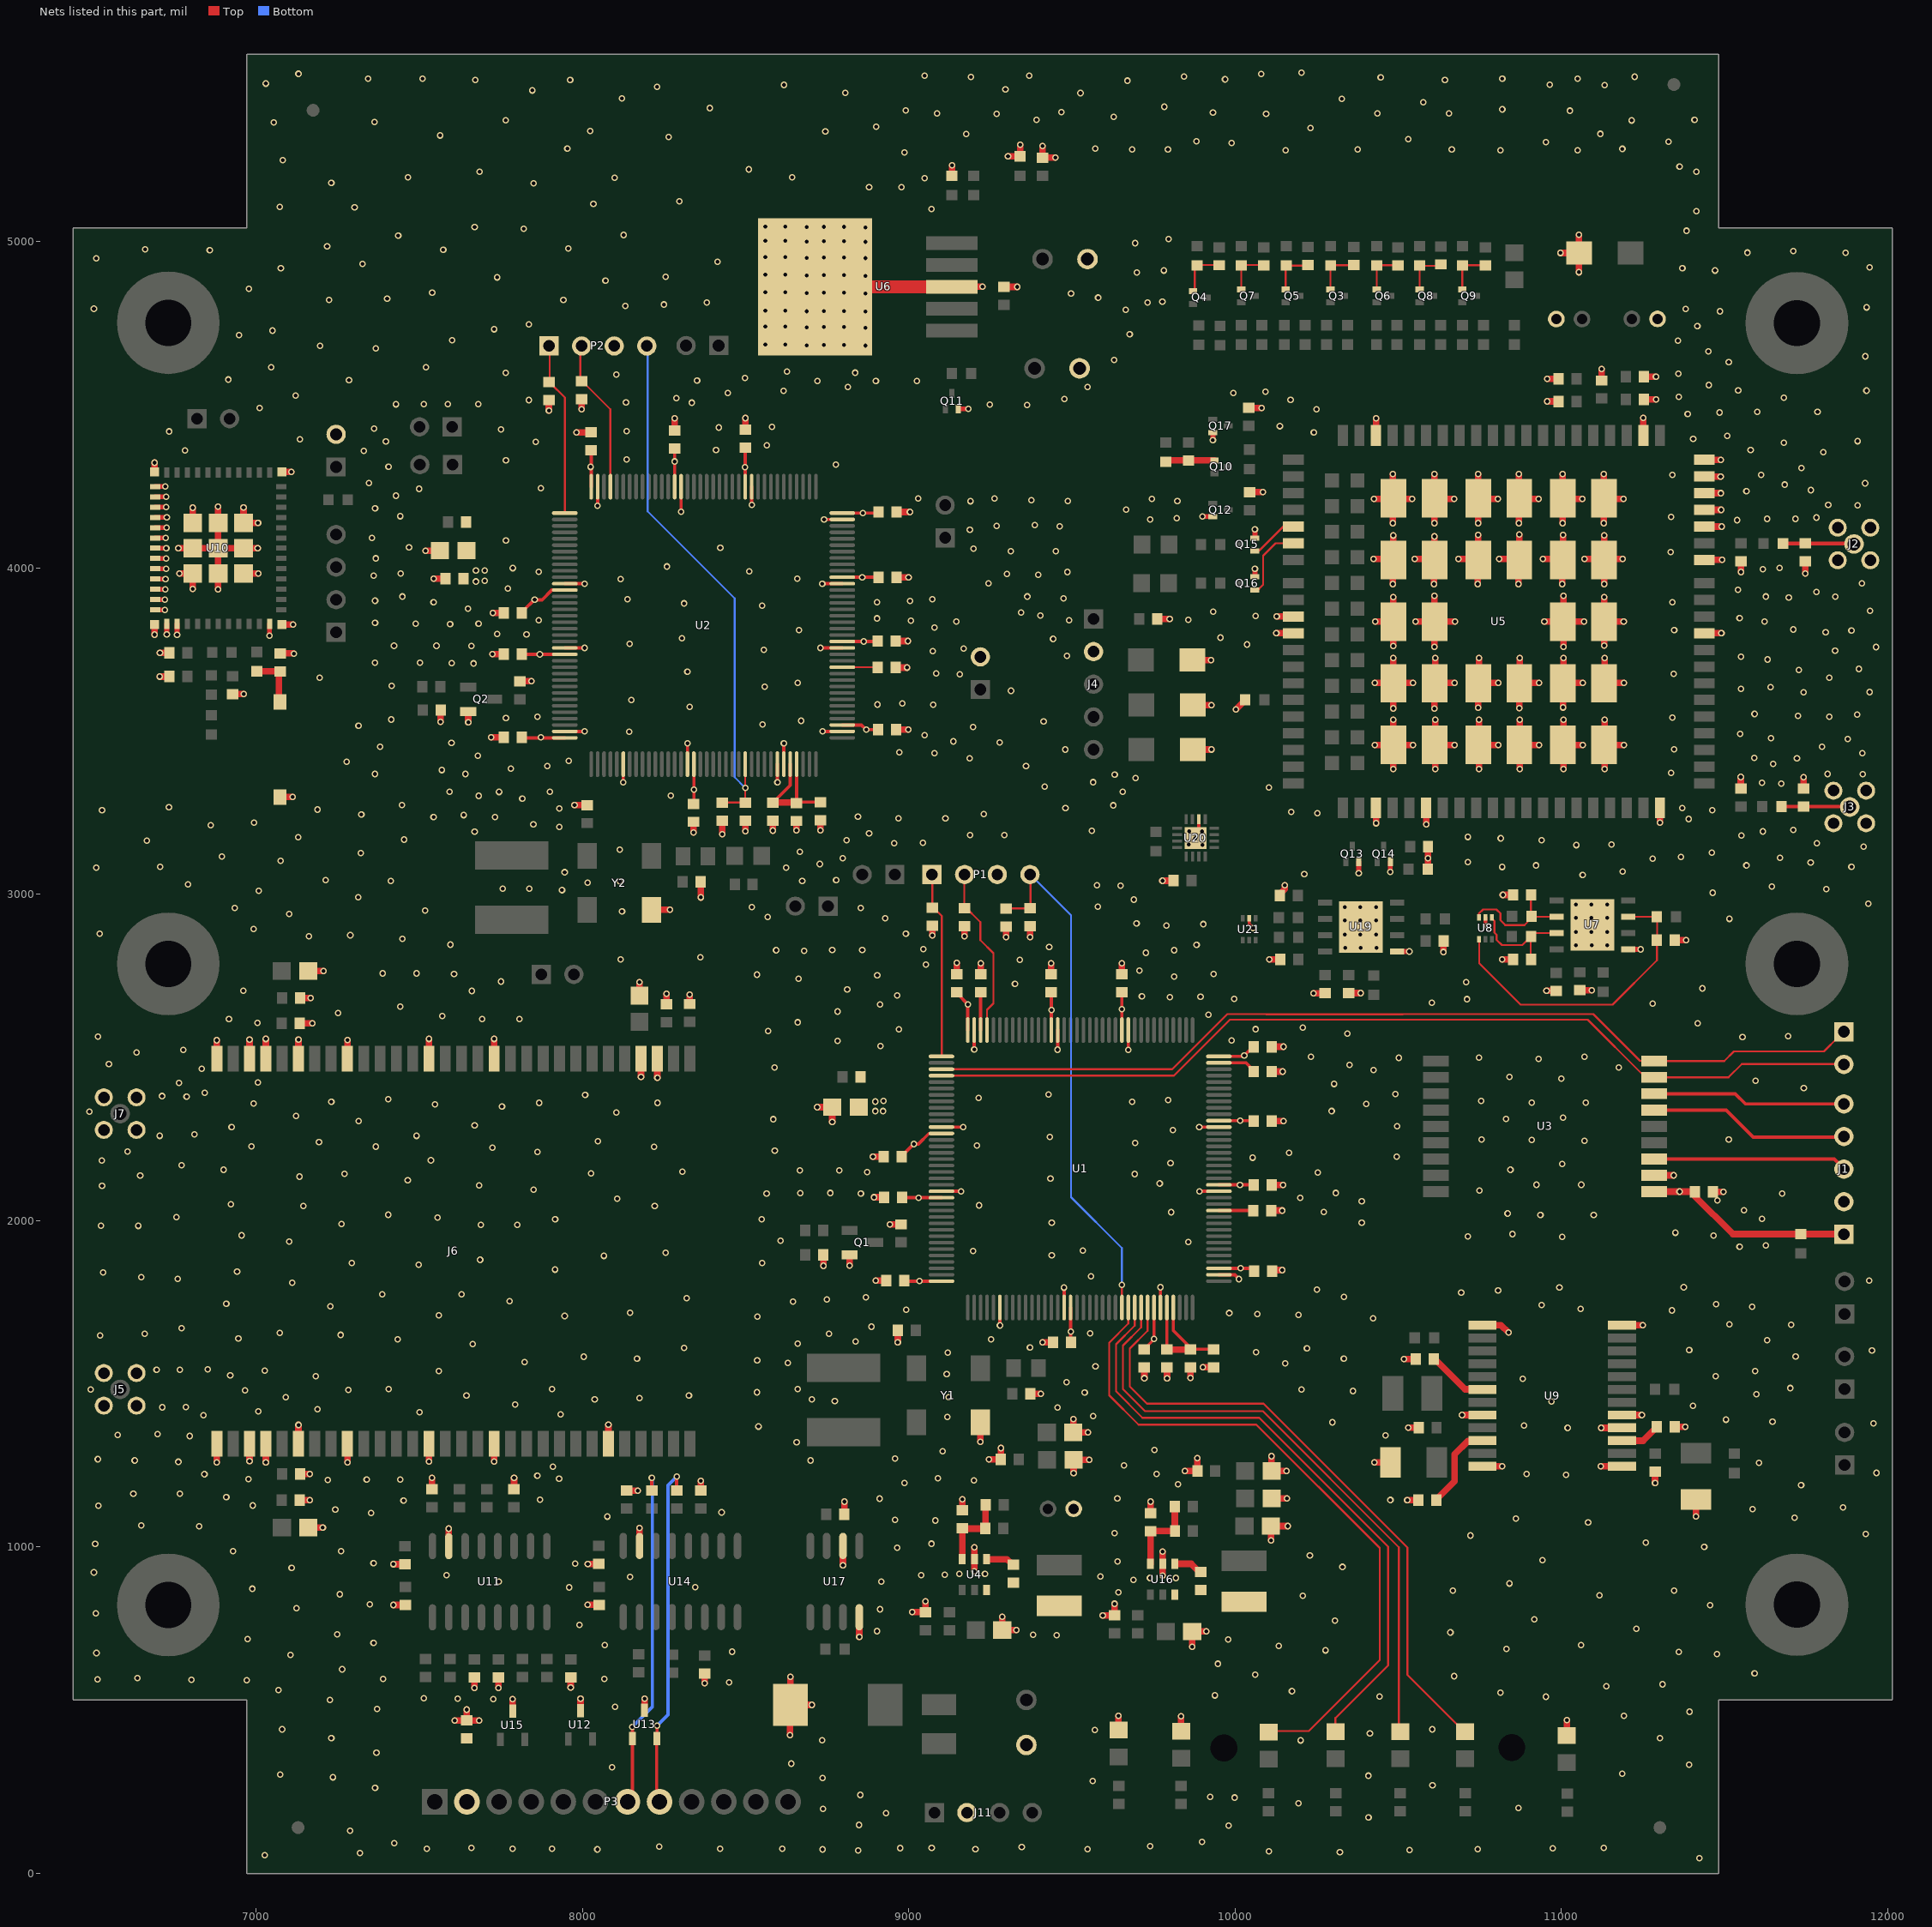
[diagram p0: the nets of this part, all layers, seen from the top]
# Altium PCB MISC86294.PcbDoc (part 5 of 8)
Units mil, origin at the board's own origin, x right, y up, seen from the top; angles counter-clockwise.
Board outline 5574.84 x 5574.84 mil, 4 copper layers (Top, GND02, PWR03, Bottom), stack 23.756 mil thick; 313 components, 311 nets, 1350 pads, 1701 vias.

## Via types
v1: diameter 20, hole 12, Top to Bottom, 1701 vias

## Nets (pads, with @x,y where several pads share a name; then routed paths per layer and width w, separated by ;. In a path a pad name is that pad's centre, name@x,y a point inside that pad or via, vN(x,y) a via of type N, cw(c..) or ccw(c..) an arc to the next point about the centre after c; other vN are vias at no path point) (continued)
GND: (continued)
  other v1: 11423,46 7026,55 7318,62 10321,65 10104,67 8845,70 10535,71 8045,73 8735,73 9204,74 9548,74 10744,74 7522,75 7785,75 7906,75 8421,75 8612,75 10974,76 8973,77 7659,78 9070,78 11130,78 9346,80 8235,82 9740,83 7423,92 9899,96 7287,130 9980,146 8847,148 10409,171 8930,184 8737,197 10868,200 10194,214 9998,232 9924,234 8851,240 7364,262 10605,270 9563,283 8735,292 7235,294 10408,299 7073,302 11186,305 8090,325 11391,333 8640,336 7368,369 10201,407 8734,408 7230,414 11302,414 10413,429 9570,439 7079,441 10604,441 11192,482 11393,495 7370,503 8099,510 7226,531 7726,534 7617,535 7513,536 10953,541 10443,542 9938,545 10813,553 10174,558 7068,561 11138,573 11310,579 8449,585 6971,592 6801,593 6513,594 7388,595 8067,595 6635,598 10671,604 10061,609 11592,613 7263,625 9947,642 7105,669 11477,672 6510,675 11360,678 8458,679 10277,683 10832,687 10134,697 8068,699 11060,699 7359,706 9979,716 6973,718 9453,730 9381,731 7248,732 10660,738 8902,742 11230,749 7990,761 10306,774 10917,778 6508,797 8912,809 7123,812 11456,821 7348,824 10207,850 11117,852 7256,855 9642,861 10667,866 11345,866 6988,872 7959,876 8345,877 10841,888 7743,894 8916,894 9688,899 9739,905 9818,905 8145,908 9587,910 7583,913 9038,913 9110,915 9155,917 9233,917 6502,922 7108,936 10329,939 7977,949 7359,950 9640,956 10942,959 10229,974 6929,987 7260,987 8964,998 11438,1000 6506,1009 9069,1010 11259,1013 10721,1035 11933,1040 9630,1042 6825,1063 6647,1066 11082,1075 9081,1081 8958,1083 10861,1087 11715,1090 8076,1093 7352,1104 8426,1106 7242,1115 11586,1116 11863,1121 6516,1126 6989,1127 7451,1142 10476,1144 7869,1145 8910,1148 9639,1149 6908,1153 6623,1163 6766,1163 11735,1189 9825,1192 8987,1196 9199,1204 7219,1205 7338,1207 7441,1207 6976,1208 7928,1209 9089,1210 7861,1218 11014,1221 6841,1223 9759,1224 10893,1224 11966,1227 7909,1246 9659,1250 11606,1258 6761,1261 6627,1265 8699,1265 6514,1269 8958,1271 9103,1293 9753,1297 8656,1321 6796,1340 10461,1342 6575,1343 6697,1346 11019,1365 8539,1369 10886,1372 11957,1379 10298,1382 11647,1384 11504,1390 9118,1398 9565,1401 6838,1404 7933,1406 7500,1413 7006,1416 7187,1422 9456,1427 6712,1428 6784,1429 11403,1433 7793,1437 10970,1446 8773,1447 8037,1452 8703,1452 8174,1456 7090,1459 9122,1459 7644,1464 8326,1464 11598,1468 9539,1473 8534,1474 10361,1478 6965,1480 7282,1481 6492,1483 10203,1483 7406,1484 7906,1484 8659,1484 11702,1487 9483,1505 10882,1515 7182,1523 11473,1523 6920,1526 9116,1530 7559,1539 11594,1539 7026,1540 6694,1543 6766,1543 6851,1544 9572,1554 10153,1563 8629,1564 7822,1567 8535,1572 8167,1577 10333,1577 8003,1583 11718,1584 9119,1596 10064,1597 11952,1602 11392,1603 10220,1609 8311,1610 9371,1611 7663,1622 8659,1623 8837,1630 11631,1634 7433,1636 9252,1636 6945,1639 6521,1648 7258,1650 6658,1653 8755,1653 9556,1655 7072,1656 6771,1670 8885,1675 11704,1681 11515,1682 10423,1701 8536,1706 7945,1708 7559,1710 10194,1711 10068,1714 9982,1717 8145,1718 11339,1725 8992,1727 11059,1730 11585,1736 7227,1737 10939,1741 11474,1744 6908,1745 8645,1752 7776,1753 8749,1759 8319,1762 8868,1765 10334,1766 7386,1774 7629,1774 10693,1780 10806,1786 10251,1789 10994,1795 11375,1796 7110,1810 11943,1816 6759,1822 6647,1827 9558,1830 6530,1841 6941,1844 7915,1850 7498,1865 7293,1870 8550,1870 7686,1880 8065,1892 9438,1894 8255,1902 9197,1907 9533,1908 11546,1920 11627,1924 9856,1935 7101,1936 8607,1939 11002,1950 10713,1952 11466,1954 6955,1955 10850,1959 11349,1963 6638,1984 6524,1985 7688,1987 7800,1987 7261,1990 9438,1994 10388,1994 7916,2004 8549,2004 11615,2006 7555,2010 6755,2011 10936,2017 11099,2017 7404,2018 10835,2022 9804,2026 10272,2027 11560,2032 7144,2045 8221,2045 9215,2047 6922,2050 10388,2059 11478,2062 8106,2067 10199,2070 8564,2083 8853,2083 11677,2083 8667,2084 8759,2085 10309,2085 10749,2092 7850,2095 6527,2107 7683,2108 10924,2110 11061,2110 9769,2114 7464,2124 9434,2129 7132,2135 6644,2138 9692,2143 7270,2144 8026,2145 10253,2148 8872,2149 8306,2150 8666,2154 8787,2154 6900,2156 10844,2156 6771,2170 11002,2174 9802,2176 6526,2184 7535,2185 10054,2193 10495,2196 10165,2208 7862,2211 6605,2212 8589,2215 7724,2224 8219,2226 7366,2227 6985,2228 9209,2230 9694,2238 7192,2241 8047,2243 11071,2245 10909,2247 10755,2249 11513,2249 9432,2257 6704,2260 7491,2260 6810,2264 9809,2278 6924,2287 10496,2289 7669,2292 7314,2305 8584,2311 10830,2312 11005,2316 7122,2321 8103,2331 6488,2334 10296,2336 7753,2350 7547,2356 10402,2358 6992,2359 7867,2361 8230,2361 10909,2362 11075,2362 7230,2364 9684,2364 10754,2367 9795,2370 7404,2372 9214,2376 6786,2380 6711,2382 8008,2385 9428,2387 10491,2388 6842,2392 11743,2406 10303,2419 6763,2422 7005,2423 11595,2429 11000,2435 10841,2441 10424,2462 6833,2466 8588,2469 11176,2470 10351,2477 6548,2480 10930,2496 10502,2499 10747,2500 10232,2502 11071,2502 6633,2515 6776,2523 8913,2535 8781,2551 9989,2552 11555,2563 6515,2564 11695,2565 10344,2573 8569,2581 8969,2586 10063,2587 10207,2592 11418,2605 7003,2606 8659,2608 6916,2618 7692,2618 7806,2618 7570,2627 9918,2631 7250,2636 8781,2641 7441,2656 8912,2663 11280,2665 10603,2668 10711,2679 9997,2680 9800,2685 9894,2686 9714,2688 8964,2690 7660,2704 6960,2705 8811,2709 11432,2712 9325,2726 10708,2731 7750,2733 8662,2742 9813,2748 8903,2752 8534,2754 7606,2756 9934,2756 7387,2758 7491,2758 9707,2767 9052,2785 9340,2799 8116,2801 8361,2807 9726,2821 8679,2827 8593,2829 9813,2829 8765,2830 8857,2830 9044,2832 10337,2836 10385,2836 10433,2836 9430,2839 11045,2844 11093,2844 11141,2844 9882,2845 7595,2846 7448,2864 7161,2872 7288,2875 10336,2877 10384,2877 10432,2877 6520,2880 8991,2880 11044,2885 11092,2885 11140,2885 6992,2894 9789,2904 9903,2909 9698,2911 10336,2920 10384,2920 10432,2920 11515,2925 8927,2927 11044,2928 11092,2928 11140,2928 8567,2931 7101,2940 8121,2948 7517,2951 6934,2958 8852,2958 8519,2961 10336,2961 10384,2961 10432,2961 9579,2962 11044,2969 11092,2969 11140,2969 11941,2972 9690,2984 7312,2991 11464,3005 7007,3011 7937,3013 11812,3016 7837,3017 7755,3018 11645,3024 9649,3027 9577,3028 6790,3031 8015,3036 8114,3040 7412,3041 8673,3041 7212,3044 8777,3044 11065,3060 10212,3062 7945,3068 11188,3070 6509,3082 8624,3082 10818,3084 6705,3085 11889,3085 10922,3089 11567,3089 8727,3093 11764,3098 10713,3099 7074,3103 11280,3110 8797,3111 11670,3112 11366,3115 6894,3116 7320,3127 11461,3128 8666,3131 8114,3137 11926,3146 11046,3151 9900,3152 9858,3153 11154,3153 8955,3157 11783,3157 9043,3158 6664,3165 8809,3166 10939,3166 7453,3168 9878,3172 10814,3172 7128,3175 10713,3176 11552,3180 9188,3182 9293,3182 8878,3187 7669,3192 9898,3193 11618,3193 9859,3194 9561,3195 11711,3198 7929,3207 6860,3212 7849,3215 6993,3220 11390,3231 8968,3233 9112,3233 7543,3237 7731,3237 8844,3238 7636,3243 7322,3245 9230,3246 10252,3249 10172,3253 6527,3258 11462,3258 7187,3260 7929,3263 9480,3265 11370,3265 6732,3267 9626,3273 7446,3274 7815,3293 7682,3302 8270,3303 7744,3314 7592,3315 7900,3315 9655,3315 10104,3328 9416,3330 11674,3339 11615,3342 9565,3344 9695,3357 9631,3367 11924,3368 7363,3369 7641,3369 11816,3369 11336,3372 7568,3381 7780,3385 7892,3393 9359,3393 11649,3400 7277,3406 7957,3409 9186,3417 11722,3417 11591,3418 7679,3425 9079,3433 11922,3433 8971,3435 9479,3444 11345,3445 7379,3452 11799,3453 7598,3464 9278,3466 9136,3469 11878,3476 11642,3479 9048,3488 11548,3492 8143,3499 9197,3513 7313,3517 8552,3521 9413,3530 8670,3532 7413,3536 7765,3541 11340,3542 7862,3545 11821,3545 11725,3547 11907,3551 11592,3553 8328,3575 9075,3581 8904,3582 8980,3585 8149,3596 11742,3619 11945,3620 9313,3624 11550,3630 11641,3635 8558,3637 7415,3639 8659,3648 7194,3664 11821,3664 9156,3675 11344,3676 9084,3677 8321,3682 11728,3688 11912,3691 7666,3708 7599,3709 7363,3710 7501,3710 11632,3720 11550,3728 9485,3731 7115,3738 9073,3746 11839,3747 8555,3749 9168,3753 11964,3758 7659,3761 7422,3762 7552,3762 10037,3766 8144,3768 9442,3783 8304,3785 9955,3787 7828,3797 7738,3798 11810,3803 11889,3809 8663,3810 11346,3810 11711,3812 9078,3818 7594,3828 7488,3830 7681,3830 7364,3832 9146,3836 11623,3836 9006,3839 7866,3840 9491,3840 9856,3841 8902,3846 11546,3847 10063,3853 9403,3855 9344,3864 9933,3866 11946,3869 7649,3876 8550,3885 8311,3892 7543,3895 8902,3895 11340,3895 9004,3899 7364,3900 8138,3905 9072,3905 9474,3907 11697,3910 11840,3912 7448,3913 9363,3913 11627,3913 11782,3927 11541,3934 7771,3937 9244,3953 11921,3953 8116,3966 8658,3968 7360,3977 9397,3980 9301,3982 7442,3983 9486,3988 7865,3989 8511,3990 11617,3997 7786,4000 11669,4001 8258,4005 7366,4030 11335,4049 9312,4052 9450,4052 9198,4060 8422,4062 7468,4064 7765,4085 7354,4093 9187,4117 9462,4128 9269,4129 9386,4132 11539,4147 9740,4149 11631,4151 11717,4151 9821,4153 11782,4155 11336,4157 7441,4159 9666,4179 7364,4183 11908,4192 11818,4194 9189,4205 9487,4206 9823,4206 9376,4208 9745,4212 9029,4213 9262,4213 7428,4222 11567,4236 11765,4239 7499,4243 7872,4245 11685,4256 11931,4260 7345,4261 11340,4286 11612,4286 11736,4307 7405,4311 8776,4317 7765,4330 8135,4333 11803,4355 7329,4359 6781,4361 8409,4362 11580,4362 8565,4376 11682,4384 7856,4387 7397,4388 11908,4389 7134,4395 11404,4396 11508,4405 10241,4416 6733,4419 8135,4420 7750,4425 7361,4428 8417,4431 8580,4433 10137,4435 11387,4472 11485,4477 11600,4479 11785,4479 10249,4487 7010,4491 9362,4500 9248,4501 7428,4502 7513,4503 7587,4503 7680,4503 8335,4507 8133,4508 7835,4515 10170,4516 9477,4518 8287,4521 11682,4522 11360,4525 7120,4529 8445,4537 9994,4537 10093,4541 8616,4543 11935,4544 11542,4545 8813,4555 9548,4555 11452,4561 8720,4574 8899,4574 9025,4574 8351,4575 7284,4576 6914,4578 8498,4583 8103,4593 11359,4596 7764,4598 8835,4599 8626,4602 7045,4616 7520,4616 11513,4631 9629,4638 11932,4649 11451,4664 7366,4673 7195,4681 8867,4682 8687,4683 8740,4684 8801,4684 8560,4685 8621,4685 11357,4697 7600,4698 6947,4714 9677,4717 7049,4728 7729,4732 8867,4737 8687,4738 8740,4739 8801,4739 8560,4740 8621,4740 11417,4742 7835,4747 8867,4786 8687,4787 11486,4787 8740,4788 8801,4788 8560,4789 8621,4789 9665,4792 11381,4794 6502,4795 11936,4799 8131,4803 8249,4808 8381,4814 9732,4814 9777,4817 7223,4822 7941,4822 7401,4826 9580,4829 8867,4842 9497,4842 8687,4843 7539,4844 8740,4844 8801,4844 8560,4845 8621,4845 6977,4856 8070,4881 7738,4891 8254,4893 8867,4896 8687,4897 8740,4898 8801,4898 8560,4899 8621,4899 9699,4906 9782,4912 11471,4912 7075,4919 11371,4919 11945,4922 7325,4932 8414,4939 6509,4949 8867,4950 8687,4951 8740,4952 8801,4952 8560,4953 8621,4953 11871,4966 11570,4967 11711,4972 6857,4974 7573,4976 6659,4977 7956,4980 7217,4986 9694,4996 8867,5000 8687,5001 8740,5002 8801,5002 8560,5003 8621,5003 9796,5008 7435,5019 8126,5021 11384,5034 7820,5040 8867,5044 7669,5045 8687,5045 8740,5046 8801,5046 8560,5047 8621,5047 11414,5094 9069,5100 7301,5106 7072,5107 8033,5116 8297,5124 8878,5168 8977,5168 7850,5179 7230,5181 9048,5195 8098,5196 7465,5198 8642,5198 7684,5215 11414,5215 8509,5222 11362,5231 7081,5250 8986,5274 10155,5281 10813,5281 11050,5281 9684,5283 9794,5283 10376,5283 10664,5283 11187,5285 7953,5286 9571,5286 9989,5303 10953,5305 11328,5307 9881,5308 10531,5315 8264,5321 7563,5326 9176,5330 11119,5331 8744,5338 8023,5340 10231,5349 8900,5353 7053,5366 7362,5367 11215,5372 7764,5373 9391,5374 11408,5374 9628,5383 9269,5392 10095,5392 9086,5394 10436,5394 10656,5394 9932,5396 9467,5398 11026,5402 8990,5403 10819,5406 8390,5410 9783,5414 10577,5428 10327,5438 8120,5440 9526,5456 8805,5457 7846,5464 9296,5467 8228,5475 11133,5480 8617,5481 10964,5482 7029,5485 9670,5494 7671,5496 7962,5496 10643,5496 9969,5498 7342,5500 7509,5500 10819,5500 11050,5500 10446,5504 9190,5505 11225,5506 9843,5507 9048,5509 9369,5509 10080,5514 7129,5515 10203,5518
GND_IN: L3.1 P3.2
GPS_DB_232RX: P3.8 R78.1 U13.2 | length 1035.6
  Top w10: P3.8@8227.15,237.85 U13.2@8227.15,412.25 ; U13.2@8228,422 v1(8228,452) ; R78.1@8288.38,1172.45 v1(8288.38,1215.38)
  Bottom w10: v1(8228,452) 8262,486 8262,1189 v1@8288,1215 ; v1@8288.38,1215 v1(8288.38,1215.38)
GPS_DB_232TX: P3.7 R76.1 U13.1 | length 1022.6
  Top w10: P3.7@8152.35,250.35 U13.1@8152.35,412.25 v1(8152.35,448.65) ; R76.1@8211.88,1172.45 v1(8211.88,1211.88)
  Bottom w10: v1(8152.35,448.65) 8214,510.3 v1@8214,1208
IMU_RST: J1.3 U3.3 | length 608
  Top w10: U3.3@11284.65,2189 11499,2189 ; 11509,2189 11499,2189 ; J1.3@11869,2156 11857,2168 11836,2189 11499,2189
IMU_RXD1: J18.1 U1.111 U3.9 | length 2919.3
  Top w6: U1.111@9099.8,2464.12 9775,2464.12 ; 9778.88,2464.12 9775,2464.12 ; U3.9@11253.5,2496.5 U3.9@11261,2489 ; U3.9@11280,2490 11241,2490 11098,2633 10514.33,2633 10513.83,2632.5 10456.17,2632.5 10095.17,2632.5 10094.67,2633 9976,2633 9807.12,2464.12 9775,2464.12 ; U3.9@11284.65,2489 11499,2489 11529,2519 11805,2519 J18.1@11849,2563
IMU_RXD2: J1.5 U3.7 | length 598.2
  Top w10: U3.7@11284.65,2389 11423,2389 ; 11438,2389 11423,2389 ; J1.5@11855,2358 11564,2358 11533,2389 11423,2389
IMU_TXD1: J18.2 U1.112 U3.8 | length 2889.8
  Top w6: U1.112@9099.8,2444.43 9812.43,2444.43 9984,2616 11081,2616 U3.8@11251,2446 ; U3.8@11284.65,2439 11512,2439 11553,2480 J18.2@11862,2480 ; U3.8@11312,2439 U3.8@11314,2441
IMU_TXD2: J1.4 U3.6 | length 633.7
  Top w10: U3.6@11284.65,2339 11405,2339 ; 11422,2339 11405,2339 ; J1.4@11867,2256 11588,2256 11505,2339 11405,2339
IMU_VDD: C35.1 J1.1 R25.2 U3.1 | length 627.8
  Top w20: U3.1@11284.65,2089 v1(11362,2089) C35.1@11405,2089 ; C35.1@11408.75,2088.89 11408.75,2075.25 11525,1959 11853,1959 J1.1@11854,1958
LED1: D14.2 U1.26 | length 2077.8
  Top w6: U1.26@9672.64,1733.8 9672.64,1684.64 9614,1626 9614,1465 9704,1375 10065,1375 10443,997 10443,653 10226,436 D14.2@10115,436
LED2: D13.2 U1.27 | length 1946.3
  Top w6: U1.27@9692.32,1733.8 9692.32,1678.32 9635,1621 9635,1477 9716,1396 10074,1396 10469,1001 10469,637 10307.52,475.52 D13.2@10307.52,433.29
LED3: D15.2 U1.28 | length 1874.9
  Top w6: U1.28@9712.01,1733.8 9712.01,1673.01 9656,1617 9656,1484 9724,1416 10085,1416 10502,999 D15.2@10502,444
LED4: D16.2 U1.29 | length 1947.7
  Top w6: U1.29@9731.69,1733.8 9731.69,1662.69 9677,1608 9677,1492 9730,1439 10087,1439 10528,998 10528,608 D16.2@10696,440
MCU1_BOOT1: R5.2 U1.48 | length 96.8
  Top w10: U1.48@9950.2,2031.05 R5.2@10046.95,2031.05
MCU1_NRST: C1.2 P1.4 R4.1 U1.25 | length 1601.6
  Top w6: C1.2@9298,2956.86 9372.86,2956.86 P1.4@9372.86,3047.14 ; U1.25@9652.95,1733.8 v1(9652.95,1803.05)
  Bottom w6: P1.4@9377,3056 9497,2936 9497,2072 9652.95,1916.05 v1(9652.95,1803.05)
MCU1_SWCLK: P1.1 R11.1 U1.109 | length 555.1
  Top w6: P1.1@9071.89,3049.89 R11.1@9071.89,2959.03 R11.1@9082.96,2947.96 ; R11.1@9085,2950 9101,2934 U1.109@9101,2508
MCU1_SWDIO: P1.2 R12.1 U1.105 | length 513.7
  Top w6: P1.2@9170,3053 9170,2964 9219,2915 9219,2860 9259,2820 9259,2666 9239.57,2646.57 U1.105@9239.57,2584.2
MCU1_VCC: C6.1 C7.1 C8.1 C9.1 C10.1 C11.1 C12.1 C13.1 C14.1 C15.1 C16.1 C17.1 C18.1 Q1.2 R1.2 R4.2 R8.1 R10.2 R12.2 U1.6 U1.17 U1.30 U1.39 U1.52 U1.62 U1.72 U1.84 U1.95 U1.108 U1.121 U1.131 U1.144 | length 1551.9
  Top w10: C13.1@8986.58,2070.42 v1@9028,2070.42 ; C14.1@8987,2207 9012.5,2232.5 v1(9015,2235) v1@9016,2236 ; C11.1@8993.49,1814.51 v1@9033,1814.51 ; v1@9017,2235 9029,2235 9061.27,2267.27 U1.121@9099.8,2267.27 ; v1(9029.42,2070.42) v1@9028,2070.42 ; v1(9033,1815) v1@9033,1814.51 ; U1.144@9099.8,1814.51 v1@9033,1814.51 ; U1.131@9099.8,2070.42 v1@9028,2070.42 ; C15.1@9151,2693 v1@9180.51,2663.49 ; U1.108@9180.51,2584.2 v1@9180.51,2663.49 ; v1(9180.51,2662.51) v1@9180.51,2663.49 ; U1.6@9278.94,1733.8 9278.94,1681.06 v1@9279,1681 ; U1.95@9436.42,2584.2 v1@9436.42,2645 ; C16.1@9436.42,2690.58 v1@9436.42,2645 ; v1(9437,2645.58) v1@9436.42,2645 ; C18.1@9495.47,1621.47 v1@9495.47,1660 ; U1.17@9495.47,1733.8 v1@9495.47,1660 ; v1(9496,1660) v1@9495.47,1660 ; U1.84@9652.95,2584.2 v1@9652.95,2649 ; v1(9652.95,2648.05) v1@9652.95,2649 ; C17.1@9652.95,2685.95 v1@9652.95,2649 ; C6.1@9729,1614 v1@9751.38,1636.38 ; v1(9751.38,1637.38) v1@9751.38,1636.38 ; U1.30@9751.38,1733.8 v1@9751.38,1636.38 ; U1.39@9950.2,1853.88 v1@10017,1853.88 ; U1.52@9950.2,2109.79 v1@10012,2109.79 ; U1.62@9950.2,2306.64 v1@10015,2306.64 ; U1.72@9950.2,2503.49 v1@10025.49,2503.49 ; v1(10014.79,2109.79) v1@10012,2109.79 ; v1(10015,2307) v1@10015,2306.64 ; v1(10017.12,1854) v1@10017,1853.88 ; v1(10028,2506) v1@10025.49,2503.49 ; C7.1@10045.12,1853.88 v1@10017,1853.88 ; C10.1@10047,2525 v1@10025.49,2503.49 ; C8.1@10047.79,2109.79 v1@10012,2109.79 ; C9.1@10048.36,2306.64 v1@10015,2306.64
  Top w20: v1(8737.61,1861.61) R1.2@8737.61,1894.89 ; v1(8818.63,1862.63) Q1.2@8818.63,1895.6 ; v1(9170.89,2872.11) R12.2@9170.89,2902.14 ; v1(9371.05,2868.95) R4.2@9371.05,2902.14 ; v1(9901.25,1550.75) R8.1@9934.11,1550.75
  other v1: 9279,1679 8897,2336 8921,2336 8897,2365 8922,2367
MCU2_BOOT1: R18.2 U2.48 | length 100.8
  Top w6: U2.48@8795.81,3696.37 R18.2@8896.63,3696.37
MCU2_NRST: C19.2 P2.4 R15.1 U2.25 | length 1650.8
  Top w6: C19.2@8433,3284 8435.57,3281.44 8498.57,3281.44 8498.57,3326 v1(8498.57,3326.56) U2.25@8498.57,3399.13
  Bottom w6: P2.4@8199,4669 8199,4174 8466,3907 8466,3359.13 v1(8498.57,3326.56)
MCU2_SWCLK: P2.1 R20.1 U2.109 | length 516.4
  Top w6: P2.1@7899,4666 7899,4569 7945.42,4522.59 U2.109@7945.42,4168.81
MCU2_SWDIO: P2.2 R21.1 U2.105 | length 459.7
  Top w6: P2.2@7993,4671 7993,4579 8085.18,4486.82 U2.105@8085.18,4249.52
MCU2_VCC: C22.1 C23.1 C24.1 C25.1 C26.1 C27.1 C28.1 C29.1 C30.1 C31.1 C32.1 C33.1 C34.1 Q2.2 R13.2 R15.2 R17.1 R19.2 R21.2 U2.6 U2.17 U2.39 U2.52 U2.62 U2.72 U2.84 U2.95 U2.108 U2.121 U2.131 U2.144 | length 1484.9
  Top w10: R13.2@7565,3561 R13.2@7566,3561 ; C25.1@7816.16,3479.84 v1@7872,3479.84 ; C24.1@7821,3872 7852,3903 7876,3903 7905.59,3932.59 U2.121@7945.42,3932.59 ; C23.1@7822.26,3735.74 v1@7868,3735.74 ; v1(7868.74,3735.74) v1@7868,3735.74 ; v1(7872,3481) v1@7872,3479.84 ; U2.144@7945.42,3479.84 v1@7872,3479.84 ; U2.131@7945.42,3735.74 v1@7868,3735.74 ; v1(8025,4310.12) v1@8026.12,4309 ; U2.108@8026.12,4249.52 v1@8026.12,4309 ; C34.1@8026.12,4354.12 v1@8026.12,4309 ; v1(8124.55,3343.55) U2.6@8124.55,3399.13 ; U2.95@8282.03,4249.52 v1(8282,4327) C27.1@8282.03,4353.03 ; v1(8341,3321) v1@8341.08,3321 ; C29.1@8341.08,3287.08 v1@8341.08,3321 ; U2.17@8341.08,3399.13 v1@8341.08,3321 ; v1(8498,4309) v1@8498.57,4309 ; U2.84@8498.57,4249.52 v1@8498.57,4309 ; C31.1@8498.57,4363.56 v1@8498.57,4309 ; U2.39@8795.81,3519.21 8854.79,3519.21 v1@8869,3505 ; U2.52@8795.81,3775.11 v1@8863,3775.11 ; U2.62@8795.81,3971.96 v1(8857.04,3972) ; U2.72@8795.81,4168.81 v1@8859,4168.81 ; v1(8857.04,3972) v1(8857.04,3972) ; v1(8859,4169) v1@8859,4168.81 ; v1(8862.11,3775.11) v1@8863,3775.11 ; v1(8870,3505) v1@8869,3505 ; C30.1@8899.11,3775.11 v1@8863,3775.11 ; C32.1@8899.96,3971.96 v1(8857.04,3972) ; C26.1@8900,3505 v1@8869,3505 ; C33.1@8900.81,4168.81 v1@8859,4168.81
  Top w20: v1(7564.61,3528.61) R13.2@7564.61,3564.89 ; v1(7649.44,3527.44) Q2.2@7649.44,3560.52 ; v1(7996.84,4486.84) R21.2@7996.84,4517.98 ; v1(8498.89,3194.11) R15.2@8498.89,3226.14 ; v1(8729.11,3195.89) R17.1@8729.11,3226.75
  other v1: 7853,3903 7673,3959 7700,3961 7673,3993 7700,3993
NET_MODE: Q15.1 U5.5 | length 143.5
  Top w6: Q15.1@10065,4054 10074,4054 10147.34,4127.35 U5.5@10178.08,4127.35
NET_STATUS: Q16.1 U5.6 | length 215.3
  Top w6: Q16.1@10073,3936 10086,3949 10086,4038 10124.17,4076.16 U5.6@10178.08,4076.16
NetC2_1: C2.1 U1.106 | length 116.9
  Top w10: U1.106@9219.88,2584.2 C2.1@9219.88,2701.12
NetC3_1: C3.1 U1.71 | length 109.6
  Top w10: U1.71@9950.2,2483.8 10033.2,2483.8 C3.1@10052,2465
NetC4_1: C4.1 C5.1 R8.2 U1.32 U1.33 | length 401.1
  Top w8: R8.2@9932,1605 R8.2@9934,1605
  Top w10: C5.1@9790.75,1612.25 U1.32@9790.75,1733.8 ; U1.33@9810.43,1733.8 9810.43,1663.57 9868,1606 R8.2@9932,1606
  Top w20: C5.1@9791.37,1605.25 C4.1@9853.25,1605.25
NetC20_1: C20.1 C21.1 R17.2 U2.32 U2.33 | length 387
  Top w10: C21.1@8591,3289 8636.36,3334.36 U2.32@8636.36,3399.13 ; U2.33@8656.05,3399.13 8656.05,3284.95 8658,3283 R17.2@8725,3283
  Top w20: C21.1@8582.6,3281.25 C20.1@8656.75,3281.25
NetC38_1: C38.1 L1.1 U4.6
NetC38_2: C38.2 U4.1 | length 78.3
  Top w20: U4.1@9238.4,962.24 9300.76,962.24 C38.2@9312,951
NetC39_2: C39.2 R27.1 R28.2 U4.3 | length 229.9
  Top w20: U4.3@9163.6,962.24 9163.6,1055.6 9164,1056 R27.1@9231,1056 ; R27.1@9235.14,1060.14 C39.2@9235.14,1129.11
NetC47_1: C47.1 L4.1 U16.6
NetC47_2: C47.2 U16.1 | length 80.4
  Top w20: U16.1@9815.4,948.24 9865.76,948.24 C47.2@9887,927
NetC48_2: C48.2 R31.1 R33.2 U16.3 | length 254.4
  Top w20: U16.3@9740.6,948.24 9740.6,1048.6 9812.6,1048.6 R31.1@9814,1050 ; R31.1@9815.14,1044 C48.2@9815.14,1124.11
NetC54_2: C54.2 Q3.2 R34.1 | length 146.2
  Top w6: Q3.2@10292.06,4853.83 10292.06,4928.06 10363.94,4928.06 C54.2@10364,4928
NetC55_2: C55.2 J2.1 R36.2 | length 204.1
  Top w11.55: R36.2@11679.29,4075.43 J2.1@11883.43,4075.43
NetC57_2: C57.2 Q4.2 R35.1 | length 132.2
  Top w6: Q4.2@9876.13,4853.83 R35.1@9876.13,4925.87 ; R35.1@9884.13,4925.87 9887.26,4929 C57.2@9943,4929
NetC58_2: C58.2 Q5.2 R38.1 | length 141.4
  Top w6: Q5.2@10154.78,4853.83 10154.78,4926.78 C58.2@10223.22,4926.78
NetC63_1: C63.1 Q6.2 R45.2 | length 142.8
  Top w6: Q6.2@10434.24,4853.83 10434.24,4930.76 10437,4928 C63.1@10499,4928
NetC68_1: C68.1 Q7.2 R49.2 | length 144.2
  Top w6: Q7.2@10018.62,4853.83 10018.62,4927.62 10020,4929 10087,4929 C68.1@10088,4928
NetC69_2: C69.2 J3.1 R46.2 | length 193.1
  Top w11.55: R46.2@11680.93,3269.07 C69.2@11742.19,3269.07 J3.1@11874.07,3269.07
NetC71_1: C71.1 Q8.2 R54.2 | length 138.6
  Top w6: Q8.2@10565.41,4853.83 10565.41,4926.59 10630.41,4926.59 C71.1@10631,4926
NetC72_1: C72.1 Q9.2 R56.2 | length 136.3
  Top w6: Q9.2@10696.59,4853.83 10696.59,4922.41 10702.17,4928 C72.1@10762,4928
NetC73_1: C73.1 Q10.2 R58.2 | length 138.8
  Top w20: R58.2@9797.98,4329.98 Q10.2@9936.82,4329.98
NetC82_1: C82.1 R67.2 U7.6 U8.3 | length 362.6
  Top w6: U8.3@10747,2933 10747,2941 10760,2954 10801,2954 10813,2942 10813,2921 10828,2906 10887,2906 10907.98,2926.98 R67.2@10907.98,2931.5 ; C82.1@10905,2994 10906.5,2992.5 10906.5,2931.5 R67.2@10907.98,2931.5 ; R67.2@10907.98,2932.92 R67.2@10907.98,2931.5 ; U7.6@10984.79,2931.5 R67.2@10907.98,2931.5
NetC84_1: C84.1 R68.2 U7.7 U8.1 | length 355.9
  Top w6: U8.1@10786,2925 U8.1@10787,2924 ; U8.1@10786.68,2929.47 U8.1@10788.57,2927.57 ; U8.1@10788,2925 10795,2918 10795,2883 10801.59,2876.41 10801.59,2860.41 10817.56,2844.44 10880.44,2844.44 R68.2@10906,2870 ; C84.1@10906,2800 R68.2@10906,2870 ; R68.2@10906.98,2870.45 10906.45,2870.45 R68.2@10906,2870 ; U7.7@10984.79,2881.5 10908.5,2881.5 10906,2879 R68.2@10906,2870
NetC85_1: C85.1 R69.2 U7.3 U8.4 | length 941.7
  Top w6: U8.4@10748,2861 10748,2789 10875,2662 11157,2662 11292.75,2797.75 C85.1@11292.75,2859.89 ; U7.3@11205.26,2931.5 11258,2931.5 11293.5,2931.5 11293.5,2866.5 C85.1@11294,2866
NetC96_1: C96.1 U9.6 | length 181.7
  Top w20: C96.1@10614,1574 10704.9,1483.1 U9.6@10758.02,1483.1
NetC97_1: C97.1 U9.15 | length 113.3
  Top w20: U9.15@11185.98,1325.62 11250.62,1325.62 C97.1@11285,1360
NetC98_1: C98.1 U9.10 | length 262.8
  Top w20: C98.1@10618,1146 10673,1201 10673,1284 10714,1325 U9.10@10754,1325 ; U9.10@10754,1325.62 U9.10@10758.02,1325.62
NetC105_1: C105.1 R73.2 SW1.2 | length 160.6
  Top w20: R73.2@7001.38,3683.73 7068.73,3683.73 7068.73,3592.27 SW1.2@7070,3591